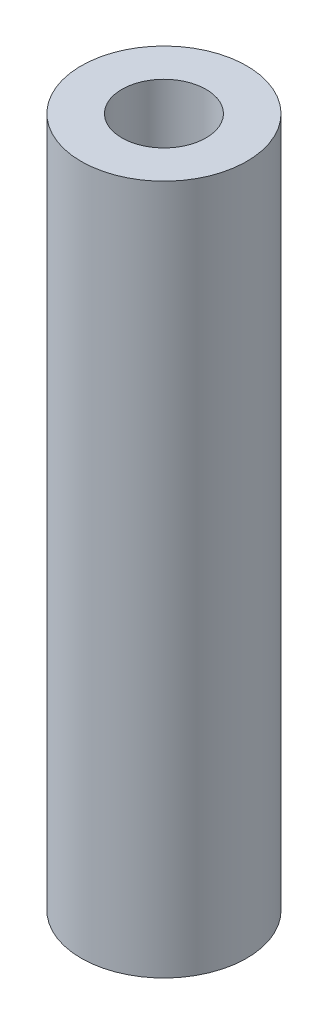
SolidWorks part; units mm, degrees
material "SS400B"
ref_plane "Front Plane" through (0, 0, 0) normal (0, 0, 1) x (1, 0, 0)
ref_plane "Top Plane" through (0, 0, 0) normal (0, 1, 0) x (1, 0, 0)
ref_plane "Right Plane" through (0, 0, 0) normal (1, 0, 0) x (0, 0, -1)
sketch "Sketch1" plane through (0, 0, 0) normal (0, 1, 0) x (1, 0, 0)
  circle A0 centre (0, 0) radius 6
  circle A1 centre (0, 0) radius 3.05
  dimension "D1" = 12
  dimension "D2" = 6.1
extrude "Boss-Extrude1" add sketch "Sketch1" along normal blind 50
